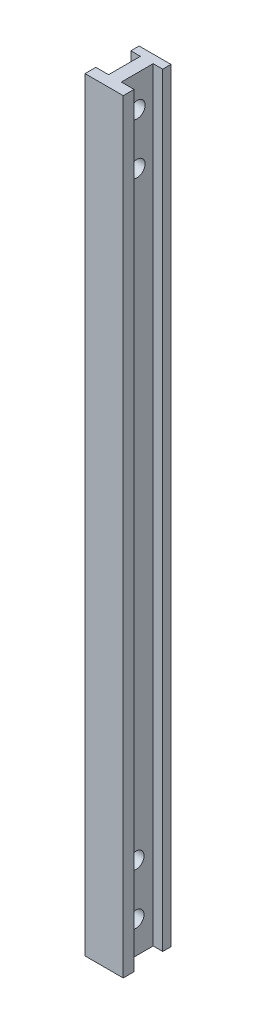
from build123d import *

# Parameters (mm, degrees)
BOSS_EXTRUDE1_DEPTH = 1200
CUT_EXTRUDE1_REACH  = 1203.333
SKETCH2_R           = 12.5


with BuildPart() as part:
    # Sketch1 → Boss-Extrude1 (new body)
    with BuildSketch(Plane(origin=(0, 0, 0), x_dir=(1, 0, 0), z_dir=(0, 1, 0))):
        Polygon((10, 27), (25, 27), (25, 40), (-25, 40), (-25, 27), (-10, 27), (-10, -23), (-30, -23), (-30, -40), (30, -40), (30, -23), (10, -23), align=None)
    extrude(amount=BOSS_EXTRUDE1_DEPTH)

    # Sketch2 → Cut-Extrude1 (cut, up to next)
    with BuildSketch(Plane(origin=(10, 0, 0), x_dir=(0, 0, -1), z_dir=(1, 0, 0)), mode=Mode.PRIVATE) as cut_extrude1_sk1:
        with Locations((1.916666667, 1150)):
            Circle(SKETCH2_R)
    cut_extrude1_tool1 = extrude(cut_extrude1_sk1.sketch, amount=-CUT_EXTRUDE1_REACH, mode=Mode.PRIVATE) & part.part
    # Sketch2 → Cut-Extrude1 (cut, up to next)
    with BuildSketch(Plane(origin=(10, 0, 0), x_dir=(0, 0, -1), z_dir=(1, 0, 0)), mode=Mode.PRIVATE) as cut_extrude1_sk2:
        with Locations((1.783333333, 1070)):
            Circle(SKETCH2_R)
    cut_extrude1_tool2 = extrude(cut_extrude1_sk2.sketch, amount=-CUT_EXTRUDE1_REACH, mode=Mode.PRIVATE) & part.part
    # Sketch2 → Cut-Extrude1 (cut, up to next)
    with BuildSketch(Plane(origin=(10, 0, 0), x_dir=(0, 0, -1), z_dir=(1, 0, 0)), mode=Mode.PRIVATE) as cut_extrude1_sk3:
        with Locations((0.083333333, 50)):
            Circle(SKETCH2_R)
    cut_extrude1_tool3 = extrude(cut_extrude1_sk3.sketch, amount=-CUT_EXTRUDE1_REACH, mode=Mode.PRIVATE) & part.part
    # Sketch2 → Cut-Extrude1 (cut, up to next)
    with BuildSketch(Plane(origin=(10, 0, 0), x_dir=(0, 0, -1), z_dir=(1, 0, 0)), mode=Mode.PRIVATE) as cut_extrude1_sk4:
        with Locations((0.216666667, 130)):
            Circle(SKETCH2_R)
    cut_extrude1_tool4 = extrude(cut_extrude1_sk4.sketch, amount=-CUT_EXTRUDE1_REACH, mode=Mode.PRIVATE) & part.part
    add(cut_extrude1_tool1.solids().sort_by_distance((10, 1150, -1.916667))[0], mode=Mode.SUBTRACT)
    add(cut_extrude1_tool2.solids().sort_by_distance((10, 1070, -1.783333))[0], mode=Mode.SUBTRACT)
    add(cut_extrude1_tool3.solids().sort_by_distance((10, 50, -0.083333))[0], mode=Mode.SUBTRACT)
    add(cut_extrude1_tool4.solids().sort_by_distance((10, 130, -0.216667))[0], mode=Mode.SUBTRACT)


solid = part.part
